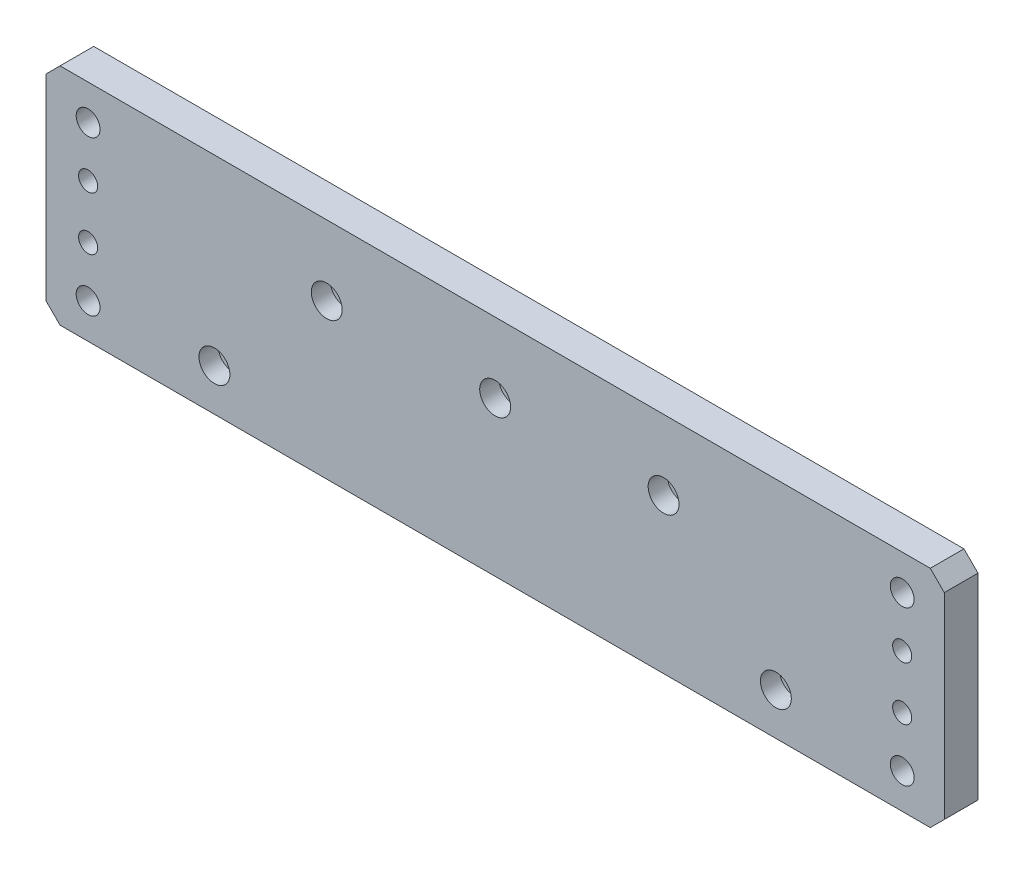
SolidWorks part; units mm, degrees
ref_plane "前视基准面" through (0, 0, 0) normal (0, 0, 1) x (1, 0, 0)
ref_plane "上视基准面" through (0, 0, 0) normal (0, 1, 0) x (1, 0, 0)
ref_plane "右视基准面" through (0, 0, 0) normal (1, 0, 0) x (0, 0, -1)
sketch "草图1" plane through (0, 0, 0) normal (0, 0, 1) x (1, 0, 0)
  line L1 (-160, 40) -> (160, 40)
  line L2 (-160, 40) -> (-160, -40)
  line L3 (-160, -40) -> (160, -40)
  line L4 (160, 40) -> (160, -40)
  line L5 (-160, 40) -> (160, -40) construction
  line L6 (-160, -40) -> (160, 40) construction
  point P0 (0, 0)
  dimension "D1" = 320
  dimension "D2" = 80
extrude "凸台-拉伸1" add sketch "草图1" along normal blind 12
chamfer "倒角1" distance 5 angle 45 4 edges at (160, -40, 6) (160, 40, 6) (-160, -40, 6) (-160, 40, 6)
hole_wizard "M8 螺纹孔1" positions "草图2" profile "草图3" tap size "M8" standard "GB" end condition through all
sketch "草图2" plane through (0, 0, 0) normal (0, 0, -1) x (-1, 0, 0)
  line L0 (0, 78.5464) -> (0, 0) construction
  line L1 (0, 0) -> (169.4504, 0) construction
  point P0 (-145, 9.5)
  point P2 (-145, -9.5)
  point P4 (145, 9.5)
  point P6 (145, -9.5)
  dimension "D1" = 290
  dimension "D2" = 19
sketch "草图3" plane through (145, 9.5, 0) normal (1, 0, 0) x (0, 1, 0)
  line L0 (0, 0) -> (0, 12)
  line L1 (0, 12) -> (3.4, 12)
  line L2 (3.4, 12) -> (3.4, 0)
  line L5 (3.4, 0) -> (0, 0)
  line L11 (0, -6.35) -> (0, 107.95) construction
  dimension "通孔螺纹孔钻头直径" = 6.8
  dimension "通孔螺纹孔钻头深度" = 12
cosmetic thread "孔螺蚊线1" parameters "D2"=8
cosmetic thread "孔螺蚊线2" parameters "D2"=8
cosmetic thread "孔螺蚊线3" parameters "D2"=8
cosmetic thread "孔螺蚊线4" parameters "D2"=8
hole_wizard "Ø8.5 (8.5) 直径孔1" positions "草图4" profile "草图5" hole size "Ø8.5" standard "GB" end condition through all
sketch "草图4" plane through (0, 0, 0) normal (0, 0, -1) x (-1, 0, 0)
  line L0 (0, 67.3739) -> (0, 0) construction
  line L1 (0, 0) -> (167.7576, 0) construction
  point P0 (-145, 27.5)
  point P2 (-145, -27.5)
  point P4 (145, 27.5)
  point P6 (145, -27.5)
  dimension "D1" = 290
  dimension "D2" = 55
sketch "草图5" plane through (145, 27.5, 0) normal (1, 0, 0) x (0, 1, 0)
  line L0 (0, 0) -> (0, 12)
  line L1 (0, 12) -> (4.25, 12)
  line L2 (4.25, 12) -> (4.25, 0)
  line L5 (4.25, 0) -> (0, 0)
  line L11 (0, -6.35) -> (0, 107.95) construction
  dimension "通孔孔直径" = 8.5
  dimension "通孔孔深度" = 12
hole_wizard "打孔尺寸(%根据)内六角圆柱头螺钉的类型1" positions "草图8" profile "草图9" counterbore size "M6" standard "GB" end condition through all
sketch "草图8" plane through (0, 0, 12) normal (0, 0, 1) x (1, 0, 0)
  line L0 (0, 0) -> (0, 92.9775) construction
  line L2 (155, 40) -> (-155, 40) construction
  point P0 (-60, 15)
  point P2 (0, 15)
  point P4 (60, 15)
  point P6 (100, -25)
  point P8 (-100, -25)
  dimension "D1" = 120
  dimension "D2" = 200
  dimension "D3" = 40
  dimension "D4" = 25
sketch "草图9" plane through (-60, 15, 12) normal (1, 0, 0) x (0, -1, 0)
  line L0 (0, 0) -> (0, 12)
  line L1 (0, 12) -> (3.3, 12)
  line L3 (3.3, 12) -> (3.3, 6.8)
  line L4 (3.3, 6.8) -> (5.5, 6.8)
  line L5 (5.5, 6.8) -> (5.5, 0)
  line L7 (5.5, 0) -> (0, 0)
  line L11 (0, -6.35) -> (0, 107.95) construction
  dimension "通孔孔直径" = 6.6
  dimension "通孔孔深度" = 12
  dimension "柱形沉头孔直径" = 11
  dimension "柱形沉头孔深度" = 6.8
